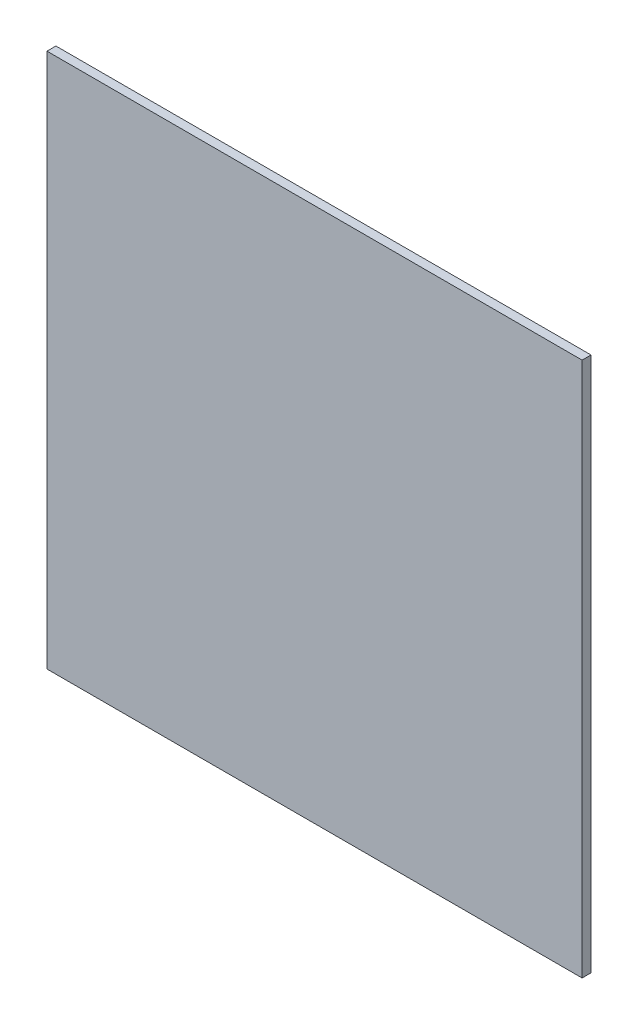
SolidWorks part; units mm, degrees
ref_plane "Front Plane" through (0, 0, 0) normal (0, 0, 1) x (1, 0, 0)
ref_plane "Top Plane" through (0, 0, 0) normal (0, 1, 0) x (1, 0, 0)
ref_plane "Right Plane" through (0, 0, 0) normal (1, 0, 0) x (0, 0, -1)
other "Configuration Table"
sketch "Sketch1" plane through (0, 0, 0) normal (0, 0, 1) x (1, 0, 0)
  line L1 (0, 0) -> (600, 0)
  line L2 (0, 0) -> (0, 600)
  line L3 (0, 600) -> (600, 600)
  line L4 (600, 0) -> (600, 600)
  dimension "D1" = 600
  dimension "D2" = 600
extrude "Boss-Extrude1" add sketch "Sketch1" along normal blind 10
